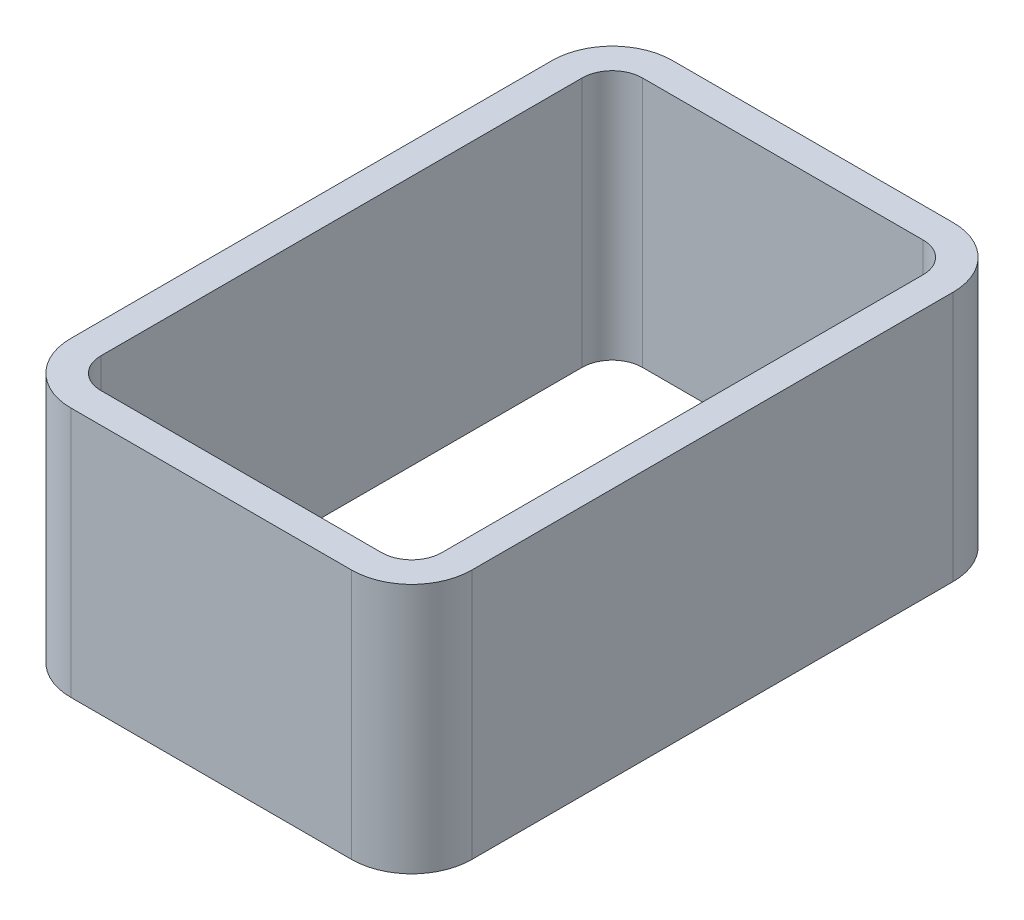
from build123d import *

# Parameters (mm, degrees)
GB_T_6728_2002_RECTANGULAR_HOLLOW_SECTIO_DEPTH = 25


with BuildPart() as part:
    # Sketch13 → GB/T 6728-2002 Rectangular Hollow Section 60X40X3(1) (new body)
    with BuildSketch(Plane(origin=(0, 0, 0), x_dir=(-1, 0, 0), z_dir=(0, 1, 0))):
        with BuildLine():
            Line((-14, -30), (14, -30))
            ThreePointArc((14, -30), (18.242640687, -28.242640687), (20, -24))
            Line((20, -24), (20, 24))
            ThreePointArc((20, 24), (18.242640687, 28.242640687), (14, 30))
            Line((14, 30), (-14, 30))
            ThreePointArc((-14, 30), (-18.242640687, 28.242640687), (-20, 24))
            Line((-20, 24), (-20, -24))
            ThreePointArc((-20, -24), (-18.242640687, -28.242640687), (-14, -30))
        make_face()
        with BuildLine():
            Line((-14, -27), (14, -27))
            ThreePointArc((14, -27), (16.121320344, -26.121320344), (17, -24))
            Line((17, -24), (17, 24))
            ThreePointArc((17, 24), (16.121320344, 26.121320344), (14, 27))
            Line((14, 27), (-14, 27))
            ThreePointArc((-14, 27), (-16.121320344, 26.121320344), (-17, 24))
            Line((-17, 24), (-17, -24))
            ThreePointArc((-17, -24), (-16.121320344, -26.121320344), (-14, -27))
        make_face(mode=Mode.SUBTRACT)
    extrude(amount=GB_T_6728_2002_RECTANGULAR_HOLLOW_SECTIO_DEPTH)


solid = part.part
